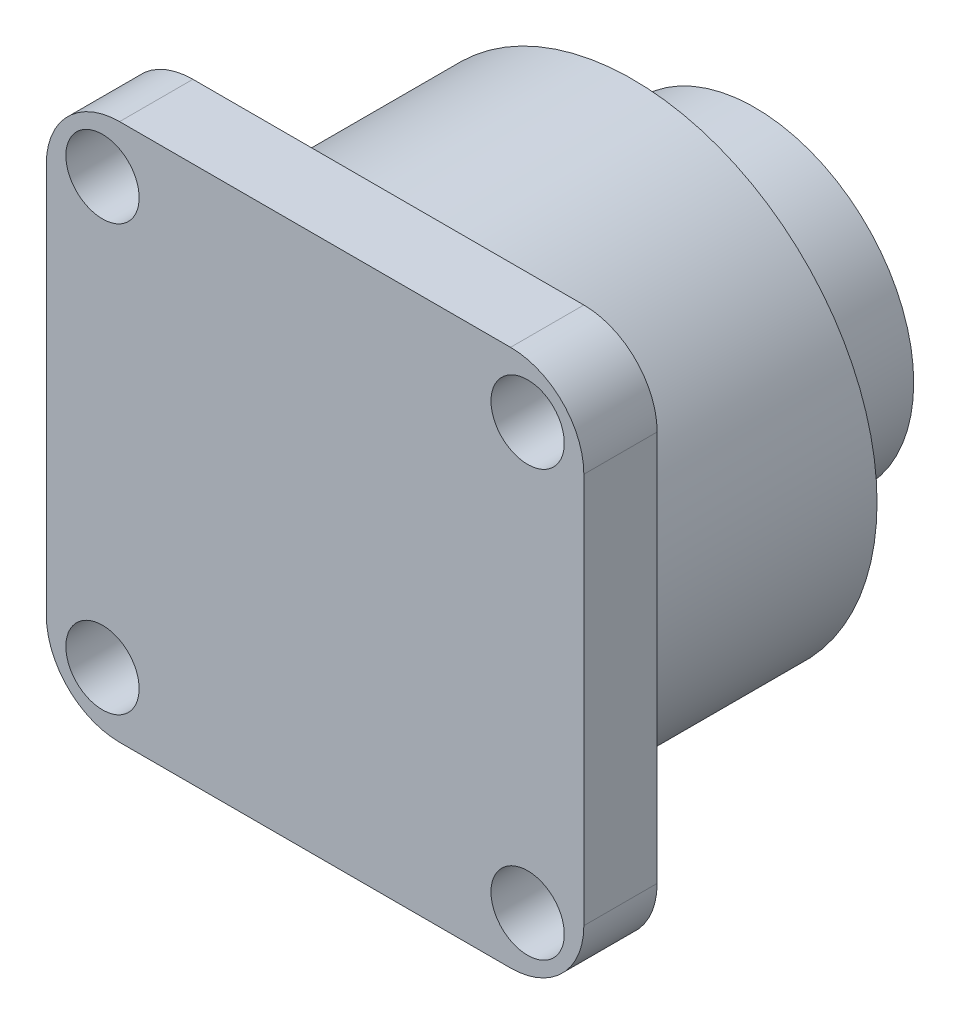
from build123d import *

# Parameters (mm, degrees)
SKETCH1_R           = 6.5
SKETCH1_R_2         = 3
BOSS_EXTRUDE1_DEPTH = 5
SKETCH2_R           = 10
BOSS_EXTRUDE2_DEPTH = 10
SKETCH3_W           = 22
SKETCH3_H           = 22
BOSS_EXTRUDE3_DEPTH = 3
FILLET1_R           = 3
SKETCH4_R           = 1.5
CUT_EXTRUDE1_DEPTH  = 3


with BuildPart() as part:
    # Sketch1 → Boss-Extrude1 (new body)
    with BuildSketch(Plane.XY):
        with Locations((-148.746139417, 0)):
            Circle(SKETCH1_R)
        with Locations((-148.746139417, 0)):
            Circle(SKETCH1_R_2, mode=Mode.SUBTRACT)
    extrude(amount=BOSS_EXTRUDE1_DEPTH)

    # Sketch2 → Boss-Extrude2 (add)
    with BuildSketch(Plane.XY.offset(5)):
        with Locations((-148.746139417, 0)):
            Circle(SKETCH2_R)
    extrude(amount=BOSS_EXTRUDE2_DEPTH)

    # Sketch3 → Boss-Extrude3 (add)
    with BuildSketch(Plane.XY.offset(15)):
        with Locations((-148.746139417, 0)):
            Rectangle(SKETCH3_W, SKETCH3_H)
    extrude(amount=BOSS_EXTRUDE3_DEPTH)

    # Fillet1
    fillet1_edges = [part.edges().sort_by_distance(p)[0] for p in [
        (-137.746139417, -11, 16.5),
        (-137.746139417, 11, 16.5),
        (-159.746139417, 11, 16.5),
        (-159.746139417, -11, 16.5),
    ]]
    fillet(fillet1_edges, radius=FILLET1_R)

    # Sketch4 → Cut-Extrude1 (cut)
    with BuildSketch(Plane(origin=(0, 0, 15), x_dir=(-1, 0, 0), z_dir=(0, 0, -1))):
        with Locations((157.446139417, 8.7)):
            Circle(SKETCH4_R)
        with Locations((157.446139417, -8.7)):
            Circle(SKETCH4_R)
        with Locations((140.046139417, -8.7)):
            Circle(SKETCH4_R)
        with Locations((140.046139417, 8.7)):
            Circle(SKETCH4_R)
    extrude(amount=-CUT_EXTRUDE1_DEPTH, mode=Mode.SUBTRACT)


solid = part.part
